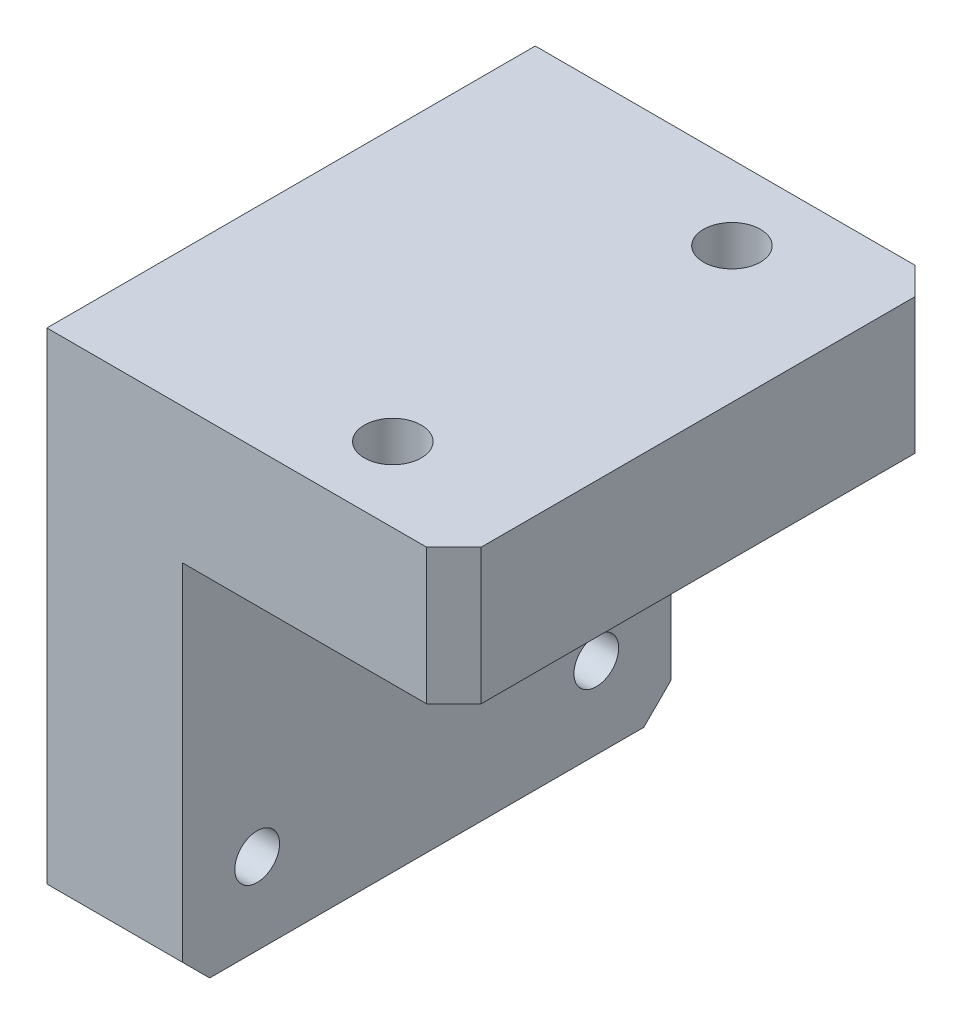
from build123d import *

# Parameters (mm, degrees)
EXTRUDE_1_DEPTH        = 18
CHAMFER_1_SIZE         = 2
HOLE_WIZARD_M4_1_D     = 3.3
HOLE_WIZARD_M4_1_DEPTH = 10.1
HOLE_WIZARD_M4_1_TIP   = 0.991420021
HOLE_WIZARD_M5_1_D     = 4.2
HOLE_WIZARD_M5_1_DEPTH = 12.4
HOLE_WIZARD_M5_1_TIP   = 1.2618073


with BuildPart() as part:
    # 草图1 → 拉伸-薄壁1 (new, symmetric)
    with BuildSketch(Plane.XY):
        Polygon((0, 0), (0, 37.5), (30, 37.5), (30, 27.5), (10, 27.5), (10, 0), align=None)
    extrude(amount=EXTRUDE_1_DEPTH, both=True)

    # 倒角1
    chamfer_1_edges = [part.edges().sort_by_distance(p)[0] for p in [
        (5, 0, 18),
        (5, 0, -18),
        (30, 32.5, -18),
        (30, 32.5, 18),
    ]]
    chamfer(chamfer_1_edges, length=CHAMFER_1_SIZE)

    # M4 螺纹孔1
    with Locations(Plane.ZY):
        with Locations((12.5, 27), (12.5, 6), (-12.5, 6), (-12.5, 27)):
            Hole(HOLE_WIZARD_M4_1_D / 2, depth=HOLE_WIZARD_M4_1_DEPTH)
            with Locations((0, 0, -(HOLE_WIZARD_M4_1_DEPTH + HOLE_WIZARD_M4_1_TIP / 2))):  # 118° drill point
                Cone(0, HOLE_WIZARD_M4_1_D / 2, HOLE_WIZARD_M4_1_TIP, mode=Mode.SUBTRACT)

    # M5 螺纹孔1
    with Locations(Plane(origin=(0, 27.5, 0), x_dir=(-1, 0, 0), z_dir=(0, -1, 0))):
        with Locations((-20, 12.5), (-20, -12.5)):
            Hole(HOLE_WIZARD_M5_1_D / 2, depth=HOLE_WIZARD_M5_1_DEPTH)
            with Locations((0, 0, -(HOLE_WIZARD_M5_1_DEPTH + HOLE_WIZARD_M5_1_TIP / 2))):  # 118° drill point
                Cone(0, HOLE_WIZARD_M5_1_D / 2, HOLE_WIZARD_M5_1_TIP, mode=Mode.SUBTRACT)


solid = part.part
